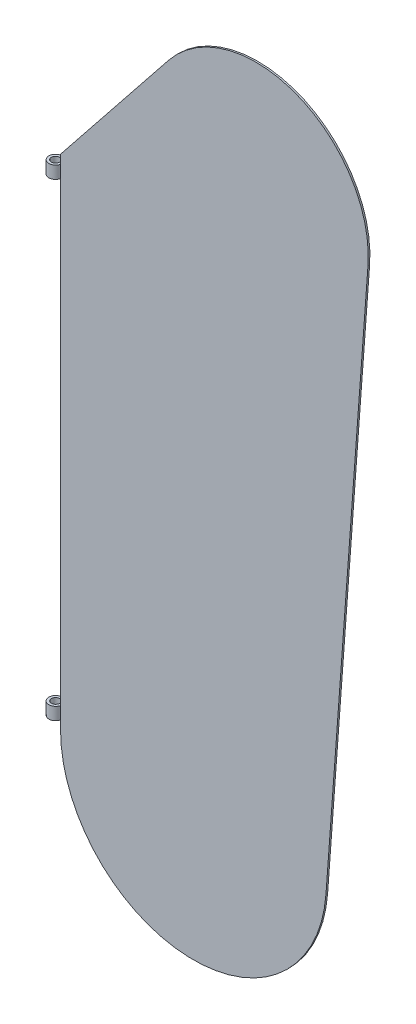
from build123d import *

# Parameters (mm, degrees)
EXTRUDE_1_DEPTH          = 2
SKETCH_2_R               = 8
EXTRUDE_2_DEPTH          = 15
SKETCH_3_R               = 8
EXTRUDE_3_DEPTH          = 15
CUT_EXTRUDE_1_DEPTH      = 776.832127461
CUT_EXTRUDE_1_DEPTH_BACK = 776.832127461
SKETCH_5_R               = 5


with BuildPart() as part:
    # 草图1 → 凸台-拉伸1 (new body)
    with BuildSketch(Plane.XY):
        with BuildLine():
            Line((134.560029616, -336.857358431), (185.128774988, 343.627300614))
            ThreePointArc((185.128774988, 343.627300614), (99.810552442, 479.304017745), (-55.008818994, 437.85123861))
            Line((-55.008818994, 437.85123861), (-185, 275))
            Line((-185, 275), (-185, -325))
            ThreePointArc((-185, -325), (-30.932759116, -484.889969571), (134.560029616, -336.857358431))
        make_face()
    extrude(amount=EXTRUDE_1_DEPTH)


with BuildPart() as body_2:
    # 草图2 → 凸台-拉伸2 (new body)
    with BuildSketch(Plane(origin=(0, -315, 0), x_dir=(1, 0, 0), z_dir=(0, 1, 0))):
        with Locations(Location((-193, 0, 0), (0, 0, 270))):
            Circle(SKETCH_2_R)
    extrude(amount=EXTRUDE_2_DEPTH)


with BuildPart() as body_3:
    # 草图3 → 凸台-拉伸3 (new body)
    with BuildSketch(Plane(origin=(0, 264.3, 0), x_dir=(1, 0, 0), z_dir=(0, 1, 0))):
        with Locations(Location((-193, 0, 0), (0, 0, 270))):
            Circle(SKETCH_3_R)
    extrude(amount=-EXTRUDE_3_DEPTH)


with BuildPart() as cut_extrude_1_tool:
    # 草图5 → 切除-拉伸1 (new, two sides: drawn at the far end of the back side and taken through both)
    with BuildSketch(Plane(origin=(0, 264.3, 0), x_dir=(1, 0, 0), z_dir=(0, 1, 0)).offset(-CUT_EXTRUDE_1_DEPTH_BACK)):
        with Locations(Location((-193, 0, 0), (0, 0, 270))):
            Circle(SKETCH_5_R)
    extrude(amount=CUT_EXTRUDE_1_DEPTH + CUT_EXTRUDE_1_DEPTH_BACK)


with BuildPart() as body_2_1:
    add(body_2.part)

    # 切除-拉伸1: cut by cut_extrude_1_tool
    add(cut_extrude_1_tool.part, mode=Mode.SUBTRACT)


with BuildPart() as body_3_1:
    add(body_3.part)

    # 切除-拉伸1: cut by cut_extrude_1_tool
    add(cut_extrude_1_tool.part, mode=Mode.SUBTRACT)


solid = Compound([part.part, body_2_1.part, body_3_1.part])
